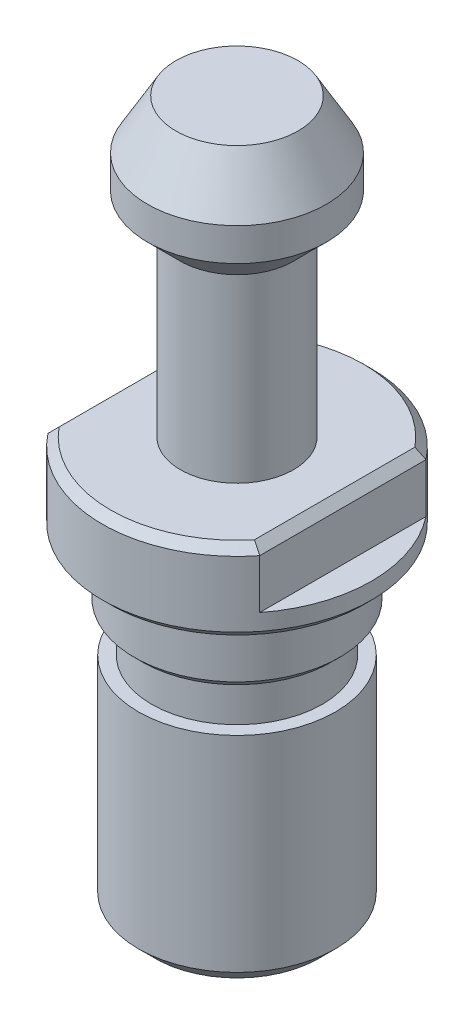
SolidWorks part; units mm, degrees
ref_plane "前视基准面" through (0, 0, 0) normal (0, 0, 1) x (1, 0, 0)
ref_plane "上视基准面" through (0, 0, 0) normal (0, 1, 0) x (1, 0, 0)
ref_plane "右视基准面" through (0, 0, 0) normal (1, 0, 0) x (0, 0, -1)
sketch "草图1" plane through (0, 0, 0) normal (0, 0, 1) x (1, 0, 0)
  line L0 (0, 43) -> (3.7179, 43)
  line L1 (3.7179, 43) -> (5.45, 40)
  line L2 (5.45, 40) -> (5.45, 38)
  line L3 (5.45, 38) -> (3.45, 36)
  line L4 (3.45, 36) -> (3.45, 25)
  line L5 (3.45, 25) -> (8.2, 25)
  line L6 (8.2, 25) -> (8.2, 20)
  line L7 (8.2, 20) -> (6.25, 20)
  line L8 (6.25, 20) -> (6.25, 16)
  line L9 (6.25, 16) -> (5.2, 16)
  line L10 (5.2, 16) -> (5.2, 13.5)
  line L11 (5.2, 13.5) -> (6, 13.5)
  line L12 (6, 13.5) -> (6, 0)
  line L13 (6, 0) -> (0, 0)
  line L14 (0, 0) -> (0, 43)
  dimension "D1" = 43
  dimension "D2" = 6
  dimension "D3" = 6.25
  dimension "D4" = 8.2
  dimension "D5" = 5.45
  dimension "D6" = 23
  dimension "D7" = 18
  dimension "D8" = 4
  dimension "D9" = 30
  dimension "D10" = 45
  dimension "D11" = 5
  dimension "D12" = 3.45
  dimension "D13" = 2.5
  dimension "D14" = 5.2
  dimension "D15" = 3
  dimension "D16" = 13.5
  dimension "D17" = 16
  dimension "D18" = 7
  dimension "D19" = 11
revolve "旋转1" add sketch "草图1" angle 360 about L14
cosmetic thread "装饰螺纹线1" parameters "D2"=10.106
chamfer "倒角1" distance 1 angle 45 1 edges at (0, 0, -6)
sketch "草图2" plane through (0, 25, 0) normal (0, 1, 0) x (1, 0, 0)
  line L0 (-8.4146, 0) -> (0, 0) construction
  line L1 (-6.45, 7.0796) -> (-10.3792, 7.0796)
  line L2 (-6.45, 7.0796) -> (-6.45, -7.0796)
  line L3 (-6.45, -7.0796) -> (-10.3792, -7.0796)
  line L4 (-10.3792, 7.0796) -> (-10.3792, -7.0796)
  line L5 (-6.45, 7.0796) -> (-10.3792, -7.0796) construction
  line L6 (-6.45, -7.0796) -> (-10.3792, 7.0796) construction
  line L7 (0, -9.02) -> (0, 9.02) construction
  line L8 (6.45, -7.0796) -> (10.3792, 7.0796) construction
  line L9 (6.45, 7.0796) -> (10.3792, -7.0796) construction
  line L10 (10.3792, 7.0796) -> (10.3792, -7.0796)
  line L11 (6.45, -7.0796) -> (10.3792, -7.0796)
  line L12 (6.45, 7.0796) -> (6.45, -7.0796)
  line L13 (6.45, 7.0796) -> (10.3792, 7.0796)
  point P0 (-8.4146, 0)
  point P14 (8.4146, 0)
  dimension "D1" = 12.9
extrude "切除-拉伸1" cut sketch "草图2" against normal blind 3.5
chamfer "倒角2" distance 0.5 angle 45 6 edges at (6.45, 25, 0) (0, 25, -8.2) (0, 25, 8.2) (-6.45, 25, 0) (0, 20, -8.2) (0, 16, -6.25)
